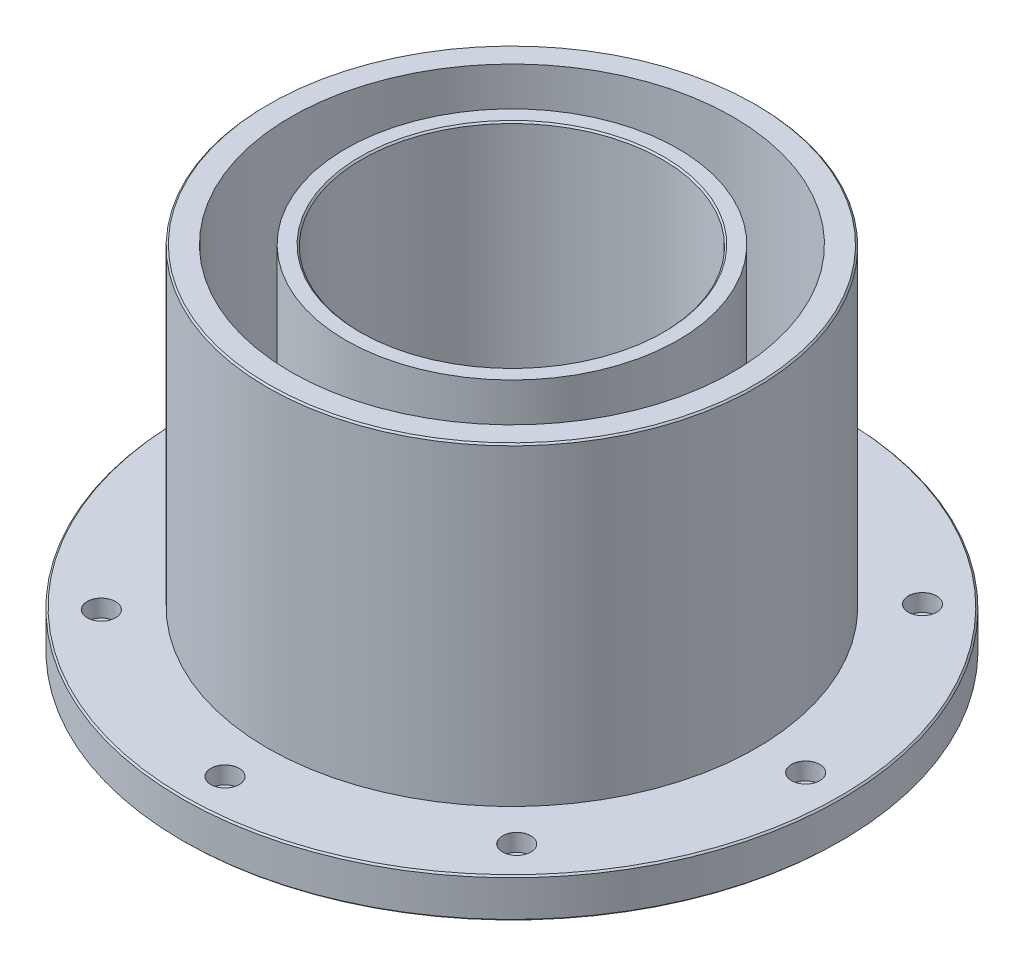
from build123d import *

# Parameters (mm, degrees)
SKETCH_1_R               = 210
EXTRUDE_1_DEPTH          = 25
SKETCH_2_R               = 95.82
CUT_EXTRUDE_1_DEPTH      = 154
EXTRUDE_START            = 200
SKETCH_3_R               = 155.82
SKETCH_3_R_2             = 95.82
EXTRUDE_2_DEPTH          = 200
CHAMFER_1_SIZE           = 1
SKETCH_7_R               = 140.82
SKETCH_7_R_2             = 105.82
CUT_EXTRUDE_3_DEPTH      = 200
PATTERN_CIRCULAR_2_COUNT = 8


with BuildPart() as part:
    # 草图1 → 凸台-拉伸1 (new body)
    with BuildSketch(Plane(origin=(0, 0, 0), x_dir=(1, 0, 0), z_dir=(0, 1, 0))):
        with Locations(Location((0, 0, 0), (0, 0, 270))):
            Circle(SKETCH_1_R)
    extrude(amount=EXTRUDE_1_DEPTH)

    # 草图2 → 切除-拉伸1 (cut)
    with BuildSketch(Plane(origin=(0, 25, 0), x_dir=(1, 0, 0), z_dir=(0, 1, 0))):
        with Locations(Location((0, 0, 0), (0, 0, 270))):
            Circle(SKETCH_2_R)
    extrude(amount=-CUT_EXTRUDE_1_DEPTH, mode=Mode.SUBTRACT)

    # 草图3 → 凸台-拉伸2 (add)
    with BuildSketch(Plane(origin=(0, 25, 0), x_dir=(1, 0, 0), z_dir=(0, 1, 0)).offset(EXTRUDE_START)):
        with Locations(Location((0, 0, 0), (0, 0, 270))):
            Circle(SKETCH_3_R)
        with Locations(Location((0, 0, 0), (0, 0, 270))):
            Circle(SKETCH_3_R_2, mode=Mode.SUBTRACT)
    extrude(amount=-EXTRUDE_2_DEPTH)

    # 倒角1
    chamfer_1_edges = [part.edges().sort_by_distance(p)[0] for p in [
        (0, 225, -155.82),
        (0, 225, -95.82),
        (0, 0, -210),
        (0, 25, -210),
    ]]
    chamfer(chamfer_1_edges, length=CHAMFER_1_SIZE)

    # 草图7 → 切除-拉伸3 (cut)
    with BuildSketch(Plane(origin=(0, 225, 0), x_dir=(1, 0, 0), z_dir=(0, 1, 0))):
        with Locations(Location((0, 0, 0), (0, 0, 270))):
            Circle(SKETCH_7_R)
        with Locations(Location((0, 0, 0), (0, 0, 270))):
            Circle(SKETCH_7_R_2, mode=Mode.SUBTRACT)
    extrude(amount=-CUT_EXTRUDE_3_DEPTH, mode=Mode.SUBTRACT)

    # 草图10 → M10 六角圆柱头螺钉的柱形沉头孔2 (revolve, cut)
    with BuildSketch(Plane(origin=(-184.987401502, 25, 2.159001035), x_dir=(0, 0, 1), z_dir=(1, 0, 0))):
        Polygon((0, 0), (0, 30.804733405), (5.5, 27.5), (5.5, 11), (9, 11), (9, 0.025), (9.025, 0), align=None)
    hole_wizard_m10_2 = revolve(axis=Axis((-184.987401502, 31.35, 2.159001035), (0, -1, 0)), mode=Mode.SUBTRACT)

    # 阵列(圆周)2: M10 六角圆柱头螺钉的柱形沉头孔2 ×8 about axis
    pattern_circular_2_axis = Axis((0, 0, 0), (0, 1, 0))
    for i in range(1, PATTERN_CIRCULAR_2_COUNT):
        add(hole_wizard_m10_2.rotate(pattern_circular_2_axis, i * 360 / PATTERN_CIRCULAR_2_COUNT), mode=Mode.SUBTRACT)


solid = part.part
